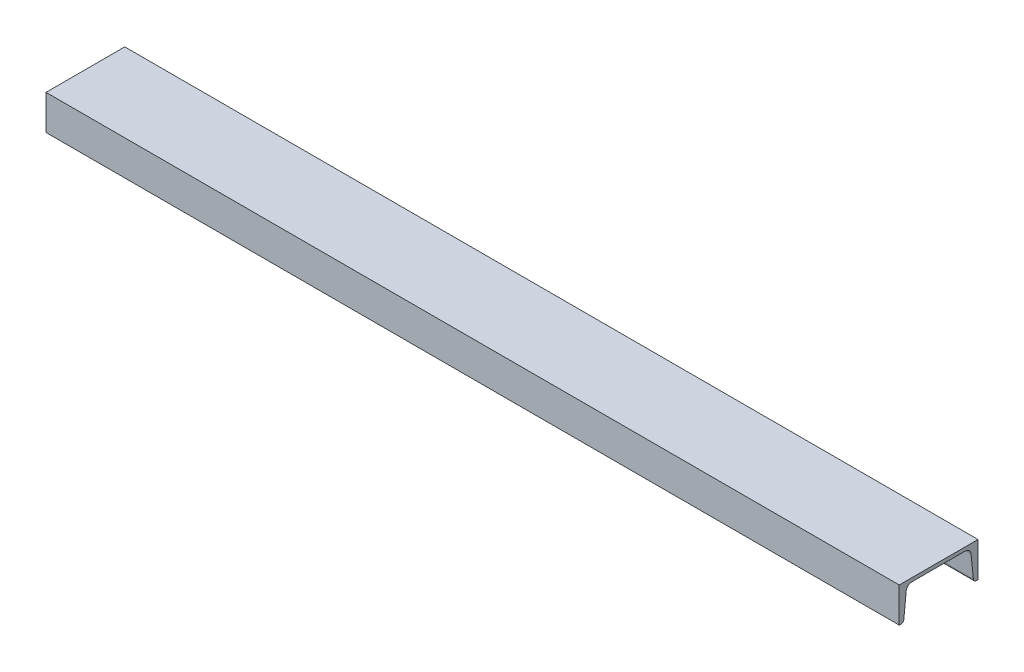
from build123d import *

# Parameters (mm, degrees)
STRUCTURAL_MEMBER1_DEPTH = 1300


with BuildPart() as part:
    # Sketch1 → Structural Member1 (new body)
    with BuildSketch(Plane.YZ.offset(-650)):
        with BuildLine():
            Line((0, 0), (0, -120))
            Line((0, -120), (-53, -120))
            Line((-53, -120), (-53, -117.44744403))
            ThreePointArc((-53, -117.44744403), (-51.836536401, -114.427920086), (-48.947766736, -112.969776674))
            Line((-48.947766736, -112.969776674), (-13.604466529, -109.435446653))
            ThreePointArc((-13.604466529, -109.435446653), (-7.826927198, -106.519159828), (-5.5, -100.480111941))
            Line((-5.5, -100.480111941), (-5.5, -19.519888059))
            ThreePointArc((-5.5, -19.519888059), (-7.826927198, -13.480840172), (-13.604466529, -10.564553347))
            Line((-13.604466529, -10.564553347), (-48.947766736, -7.030223326))
            ThreePointArc((-48.947766736, -7.030223326), (-51.836536401, -5.572079914), (-53, -2.55255597))
            Line((-53, -2.55255597), (-53, 0))
            Line((-53, 0), (0, 0))
        make_face()
    extrude(amount=STRUCTURAL_MEMBER1_DEPTH)


solid = part.part
